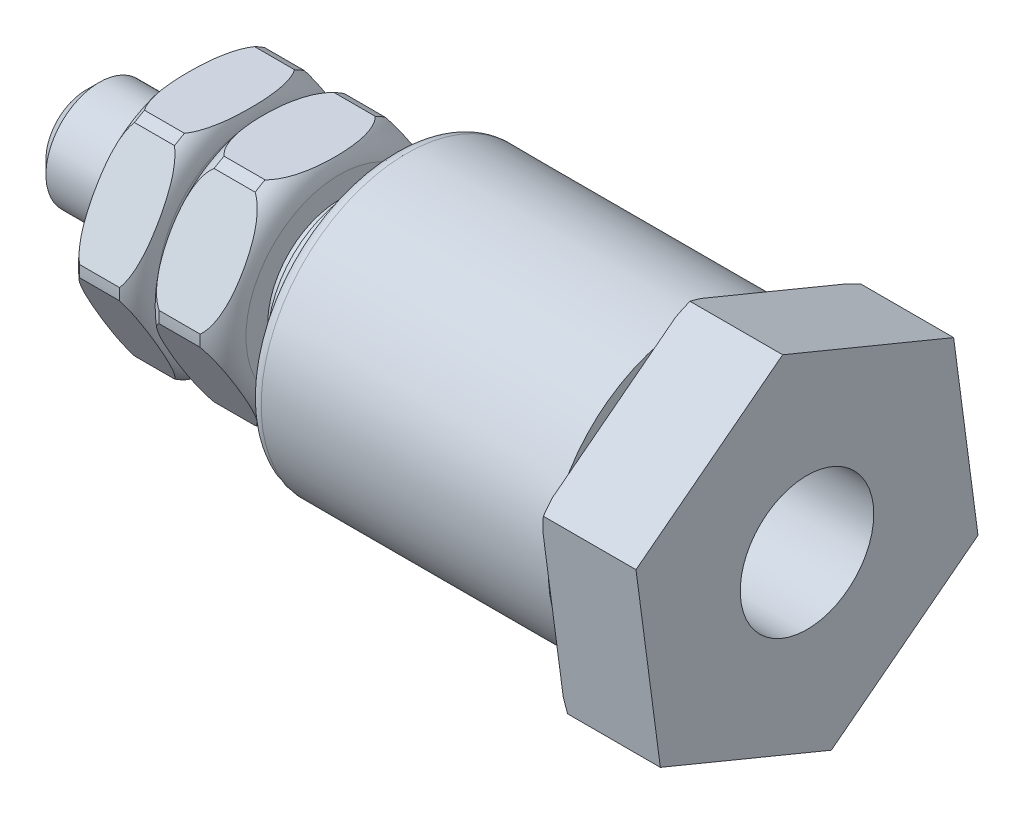
from build123d import *

# Parameters (mm, degrees)
CUT_EXTRUDE1_REACH = 53.794
SKETCH2_R          = 13.340242397
SKETCH4_OUTSIDE_W  = 48.398
SKETCH4_OUTSIDE_H  = 48.398
CUT_EXTRUDE3_DEPTH = 20


with BuildPart() as part:
    # Sketch1 → Revolve1 (revolve)
    with BuildSketch(Plane.XY, mode=Mode.PRIVATE) as revolve1_sk:
        with BuildLine():
            Line((10.553065695, 13.332305779), (10.553065695, 9.120964454))
            Line((10.553065695, 9.120964454), (9.195532772, 9.120964454))
            Line((9.195532772, 9.120964454), (9.195532772, 10.893723118))
            Line((9.195532772, 10.893723118), (-12.304467227, 10.89363247))
            ThreePointArc((-12.304467227, 10.89363247), (-13.020261836, 10.605574336), (-13.317931541, 9.893723118))
            Line((-13.317931541, 9.893723118), (-13.317931541, 9.393723118))
            Line((-13.317931541, 9.393723118), (-15.317931541, 5.393723118))
            Line((-15.317931541, 5.393723118), (-15.317931541, 6.393723118))
            Line((-15.317931541, 6.393723118), (-16.317931541, 6.393723118))
            Line((-16.317931541, 6.393723118), (-16.317931541, 5.393723118))
            Line((-16.317931541, 5.393723118), (-17.317931541, 5.393723118))
            Line((-17.317931541, 5.393723118), (-17.317931541, 7.018723118))
            ThreePointArc((-17.317931541, 7.018723118), (-17.787269372, 8.203105819), (-18.781251286, 9))
            Line((-18.781251286, 9), (-21.854611796, 9))
            ThreePointArc((-21.854611796, 9), (-23.156356824, 7.789180206), (-23.317931541, 6.018723118))
            Line((-23.317931541, 6.018723118), (-23.317931541, 5.5))
            Line((-23.317931541, 5.5), (-23.81793154, 5.5))
            Line((-23.81793154, 5.5), (-23.81793154, 7.125))
            ThreePointArc((-23.81793154, 7.125), (-24.08355654, 8.1875), (-24.81793154, 9))
            Line((-24.81793154, 9), (-27.81793154, 9))
            ThreePointArc((-27.81793154, 9), (-28.55230654, 8.1875), (-28.81793154, 7.125))
            Line((-28.81793154, 7.125), (-28.81793154, 4))
            Line((-28.81793154, 4), (-35.317931541, 4))
            Line((-35.317931541, 4), (-36.317931541, 3))
            Line((-36.317931541, 3), (-36.317931541, 0))
            Line((-36.317931541, 0), (-7, 0))
            Line((-7, 0), (-4.340647086, 5))
            Line((-4.340647086, 5), (17.682068459, 5))
            Line((17.682068459, 5), (17.682068459, 14.045862297))
            ThreePointArc((17.682068459, 14.045862297), (13.875178985, 16.110735773), (10.553065695, 13.332305779))
        make_face()
    revolve(revolve1_sk.sketch.rotate(Axis((-7, 0, 0), (-1, 0, 0)), 90), axis=Axis((-7, 0, 0), (-1, 0, 0)))

    # Cut-Extrude1: up to this face of the body (flat: up to its plane)
    cut_extrude1_end = Plane(part.part.faces().sort_by_distance((-17.317931541, 0, 5.592242587))[0])
    # Sketch2 → Cut-Extrude1 (cut, up to the picked face)
    with BuildSketch(Plane.ZY.offset(28.81793154), mode=Mode.PRIVATE) as cut_extrude1_sk1:
        Circle(SKETCH2_R)
        Polygon((-4.618802154, 8), (4.618802154, 8), (9.237604307, 0), (4.618802154, -8), (-4.618802154, -8), (-9.237604307, 0), align=None, mode=Mode.SUBTRACT)
    cut_extrude1_tool1 = split(extrude(cut_extrude1_sk1.sketch, amount=-CUT_EXTRUDE1_REACH, mode=Mode.PRIVATE), bisect_by=cut_extrude1_end, keep=Keep.BOTH, mode=Mode.PRIVATE)
    add(cut_extrude1_tool1.solids().sort_by(Axis((-28.817932, 0, -12.962923), (1, 0, 0)))[0], mode=Mode.SUBTRACT)

    # Sketch4 outside → Cut-Extrude3 (cut)
    with BuildSketch(Plane(origin=(17.682068459, 0, 0), x_dir=(0, 0, -1), z_dir=(1, 0, 0))):
        Rectangle(SKETCH4_OUTSIDE_W, SKETCH4_OUTSIDE_H)
        Polygon((12.807380528, -5.288762048), (10.983892553, 8.447135869), (-1.823487976, 13.735897918), (-12.807380528, 5.288762048), (-10.983892553, -8.447135869), (1.823487976, -13.735897918), align=None, mode=Mode.SUBTRACT)
    extrude(amount=-CUT_EXTRUDE3_DEPTH, mode=Mode.SUBTRACT)


solid = part.part
